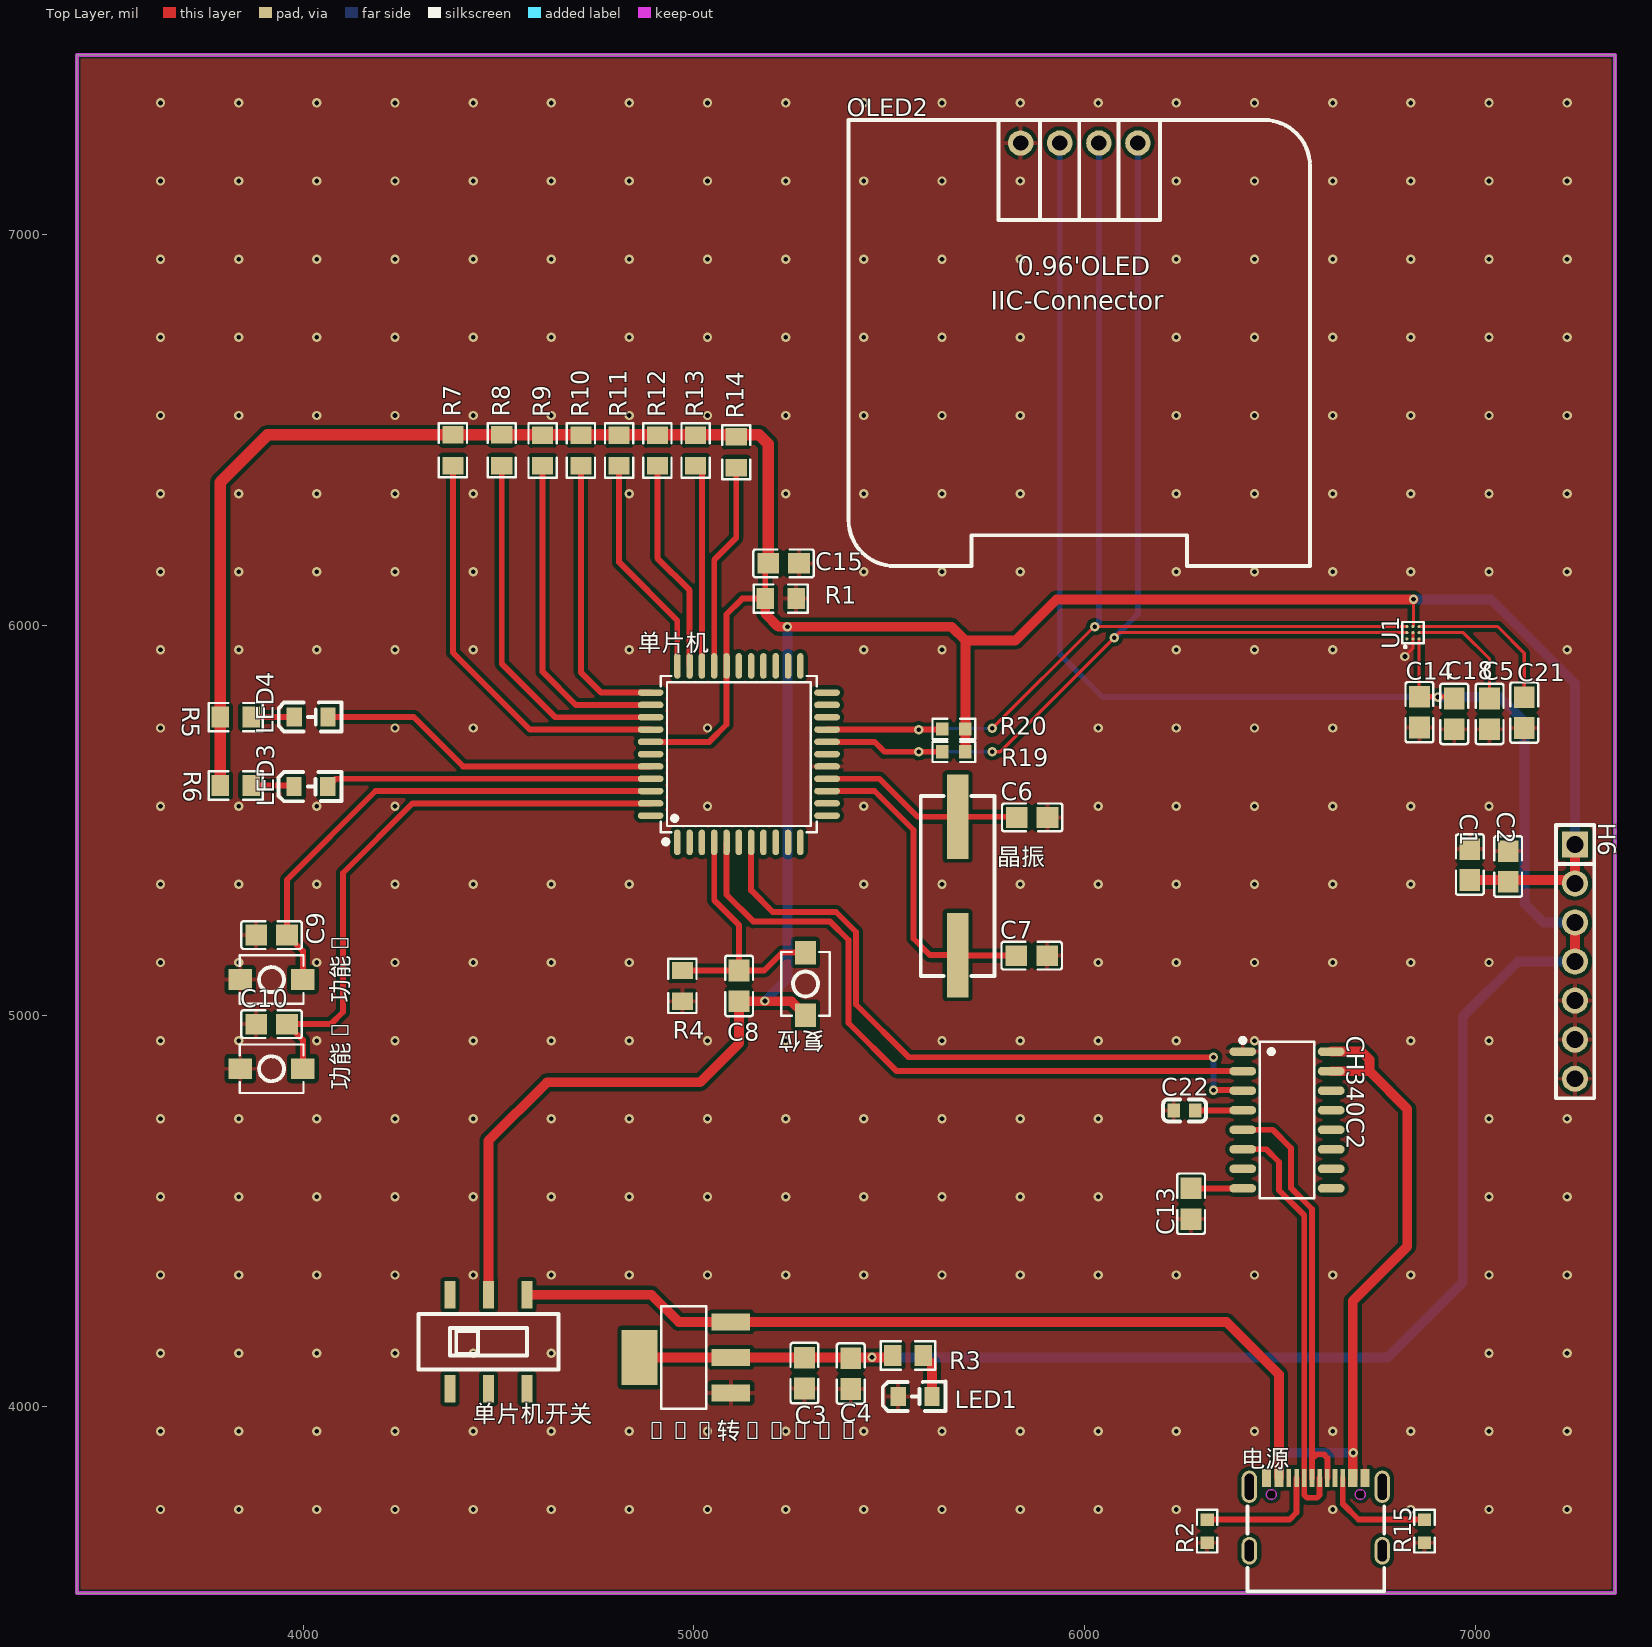
[diagram p0: Top Layer view]
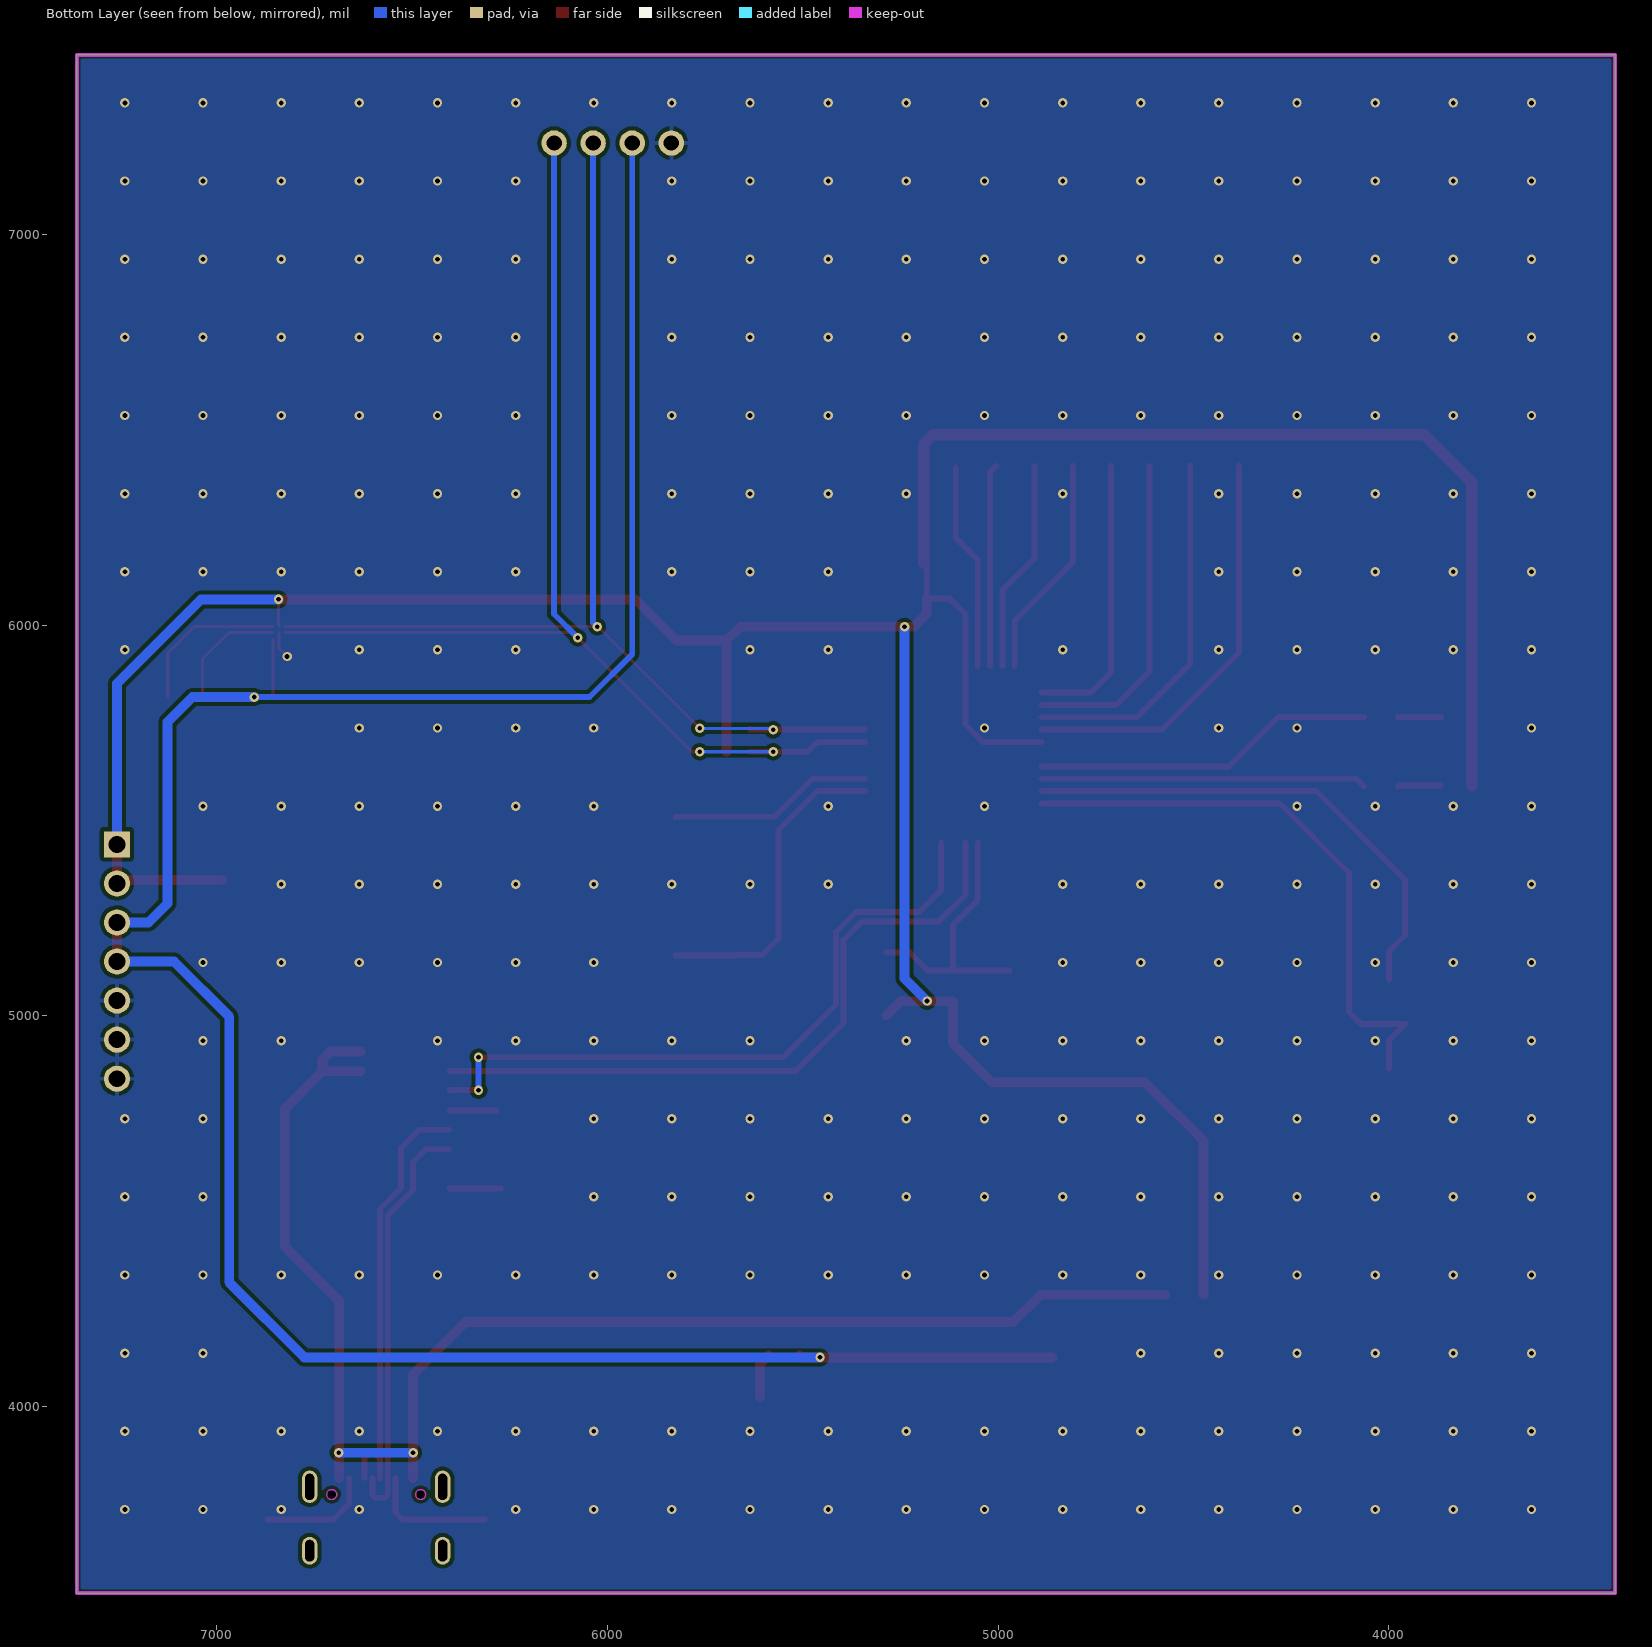
[diagram p1: Bottom Layer view, seen from below]
# Altium PCB MISC51448.pcbdoc
Units mil, origin at the board's own origin, x right, y up, seen from the top; angles counter-clockwise.
Board outline 3937.01 x 3937.01 mil, 2 copper layers (Top Layer, Bottom Layer), stack 62.206 mil thick; 48 components, 56 nets, 186 pads, 307 vias.

## Layer stack, top to bottom
Top Solder Mask Layer: solder mask 0.394, Dk 3.3
Top Layer: signal copper 1.379
Dielectric1: surface 59.449, FR4, Dk 4.5
Bottom Layer: signal copper 1.378
Bottom Solder Mask Layer: solder mask 0.394, Dk 3.3

## Board outline
3420.99,7459.65 3420.99,3522.65 7358,3522.65 7358,7459.65

## Design rules (kind name [scope] priority, off if disabled: settings)
BoardOutlineClearance copperThickness2oz_1 [All] p2 off: genericclearance=7.99 ignorepadtopadclearanceinfootprint=FALSE except(0: Arc-SplitContinuation Track-SplitContinuation SMDPad-SplitContinuation THPad-SplitContinuation Via-SplitContinuation Fill-SplitContinuation Region-SplitContinuation Poly-SplitContinuation Text-SplitContinuation Hole-SplitContinuation; 5.98: Arc-CutoutEdge SMDPad-CutoutEdge THPad-CutoutEdge Via-CutoutEdge Fill-CutoutEdge Region-CutoutEdge Text-CutoutEdge; 6.93: Hole-OutlineEdge Hole-CutoutEdge; 10: Poly-OutlineEdge Poly-CutoutEdge; 11.81: Arc-OutlineEdge Track-OutlineEdge SMDPad-OutlineEdge THPad-OutlineEdge Via-OutlineEdge Fill-OutlineEdge Region-OutlineEdge Text-OutlineEdge Track-CutoutEdge)
BoardOutlineClearance Plane_innerPlane_1 [All] p4 off: genericclearance=4.02 ignorepadtopadclearanceinfootprint=FALSE except(0: Arc-SplitContinuation Track-SplitContinuation SMDPad-SplitContinuation THPad-SplitContinuation Via-SplitContinuation Fill-SplitContinuation Region-SplitContinuation Poly-SplitContinuation Text-SplitContinuation Hole-SplitContinuation; 6: SMDPad-CutoutEdge THPad-CutoutEdge Via-CutoutEdge Fill-CutoutEdge Region-CutoutEdge Text-CutoutEdge; 6.93: Hole-OutlineEdge Hole-CutoutEdge; 10: Poly-OutlineEdge Poly-CutoutEdge; 11.8: Arc-OutlineEdge Track-OutlineEdge SMDPad-OutlineEdge THPad-OutlineEdge Via-OutlineEdge Fill-OutlineEdge Region-OutlineEdge Text-OutlineEdge; 11.81: Arc-CutoutEdge Track-CutoutEdge)
BoardOutlineClearance Copper_copperRegion_1 [All] p6 off: genericclearance=4.02 ignorepadtopadclearanceinfootprint=FALSE except(0: Arc-SplitContinuation Track-SplitContinuation SMDPad-SplitContinuation THPad-SplitContinuation Via-SplitContinuation Fill-SplitContinuation Region-SplitContinuation Poly-SplitContinuation Text-SplitContinuation Hole-SplitContinuation; 6: SMDPad-CutoutEdge THPad-CutoutEdge Via-CutoutEdge Fill-CutoutEdge Region-CutoutEdge Text-CutoutEdge; 6.93: Hole-OutlineEdge Hole-CutoutEdge; 10: Poly-OutlineEdge Poly-CutoutEdge; 11.8: Arc-OutlineEdge Track-OutlineEdge SMDPad-OutlineEdge THPad-OutlineEdge Via-OutlineEdge Fill-OutlineEdge Region-OutlineEdge Text-OutlineEdge; 11.81: Arc-CutoutEdge Track-CutoutEdge)
BoardOutlineClearance copperThickness1oz_1 [All] p8: genericclearance=4.02 ignorepadtopadclearanceinfootprint=FALSE except(0: Arc-SplitContinuation Track-SplitContinuation SMDPad-SplitContinuation THPad-SplitContinuation Via-SplitContinuation Fill-SplitContinuation Region-SplitContinuation Poly-SplitContinuation Text-SplitContinuation Hole-SplitContinuation; 6: SMDPad-CutoutEdge THPad-CutoutEdge Via-CutoutEdge Fill-CutoutEdge Region-CutoutEdge Text-CutoutEdge; 6.93: Hole-OutlineEdge Hole-CutoutEdge; 10: Poly-OutlineEdge Poly-CutoutEdge; 11.8: Arc-OutlineEdge Track-OutlineEdge SMDPad-OutlineEdge THPad-OutlineEdge Via-OutlineEdge Fill-OutlineEdge Region-OutlineEdge Text-OutlineEdge; 11.81: Arc-CutoutEdge Track-CutoutEdge)
Clearance copperThickness2oz [All] p1 off: gap=7.99 ignorepadtopadclearanceinfootprint=FALSE except(5.98: SMDPad-Track SMDPad-SMDPad THPad-Track SMDPad-THPad THPad-THPad Track-Via SMDPad-Via THPad-Via Via-Via Fill-Track Region-Track Fill-SMDPad Region-SMDPad Fill-THPad Region-THPad Fill-Via Region-Via Fill-Fill Fill-Region Region-Region Arc-Track Arc-SMDPad Arc-THPad Arc-Via Fill-Arc Region-Arc Arc-Arc Text-Track SMDPad-Text Text-THPad Text-Via Fill-Text Region-Text Arc-Text Text-Text; 6.93: Hole-Track Hole-SMDPad Hole-THPad Hole-Via Fill-Hole Region-Hole Hole-Arc Hole-Text; 10: Poly-Track Poly-SMDPad Poly-THPad Poly-Via Poly-Fill Poly-Region Poly-Poly Poly-Arc Poly-Text Poly-Hole)
Clearance Plane_innerPlane [All] p3 off: gap=4.02 ignorepadtopadclearanceinfootprint=FALSE except(4.33: SMDPad-Track SMDPad-SMDPad SMDPad-THPad; 5.98: THPad-Track THPad-THPad Track-Via SMDPad-Via THPad-Via Via-Via Fill-Track Region-Track Fill-SMDPad Region-SMDPad Fill-THPad Region-THPad Fill-Via Region-Via Fill-Fill Fill-Region Region-Region; 6: Arc-Track Arc-SMDPad Arc-THPad Arc-Via Fill-Arc Region-Arc Arc-Arc Text-Track SMDPad-Text Text-THPad Text-Via Fill-Text Region-Text Arc-Text Text-Text; 6.93: Hole-Track Hole-SMDPad Hole-THPad Hole-Via Fill-Hole Region-Hole Hole-Arc Hole-Text; 10: Poly-Track Poly-SMDPad Poly-THPad Poly-Via Poly-Fill Poly-Region Poly-Poly Poly-Arc Poly-Text Poly-Hole)
Clearance Copper_copperRegion [All] p5 off: gap=4.02 ignorepadtopadclearanceinfootprint=FALSE except(4.33: SMDPad-Track SMDPad-SMDPad SMDPad-THPad; 5.98: THPad-Track THPad-THPad Track-Via SMDPad-Via THPad-Via Via-Via Fill-Track Region-Track Fill-SMDPad Region-SMDPad Fill-THPad Region-THPad Fill-Via Region-Via Fill-Fill Fill-Region Region-Region; 6: Arc-Track Arc-SMDPad Arc-THPad Arc-Via Fill-Arc Region-Arc Arc-Arc Text-Track SMDPad-Text Text-THPad Text-Via Fill-Text Region-Text Arc-Text Text-Text; 6.93: Hole-Track Hole-SMDPad Hole-THPad Hole-Via Fill-Hole Region-Hole Hole-Arc Hole-Text; 10: Poly-Track Poly-SMDPad Poly-THPad Poly-Via Poly-Fill Poly-Region Poly-Poly Poly-Arc Poly-Text Poly-Hole)
Clearance copperThickness1oz [All] p7: gap=4.02 ignorepadtopadclearanceinfootprint=FALSE except(4.33: SMDPad-Track SMDPad-SMDPad SMDPad-THPad; 5.98: THPad-Track THPad-THPad Track-Via SMDPad-Via THPad-Via Via-Via Fill-Track Region-Track Fill-SMDPad Region-SMDPad Fill-THPad Region-THPad Fill-Via Region-Via Fill-Fill Fill-Region Region-Region; 6: Arc-Track Arc-SMDPad Arc-THPad Arc-Via Fill-Arc Region-Arc Arc-Arc Text-Track SMDPad-Text Text-THPad Text-Via Fill-Text Region-Text Arc-Text Text-Text; 6.93: Hole-Track Hole-SMDPad Hole-THPad Hole-Via Fill-Hole Region-Hole Hole-Arc Hole-Text; 10: Poly-Track Poly-SMDPad Poly-THPad Poly-Via Poly-Fill Poly-Region Poly-Poly Poly-Arc Poly-Text Poly-Hole)
DiffPairsRouting differentialPair [All] p1: maxlimit=6 minlimit=6 mostfreqgap=6 toplayer_minwidth=5 toplayer_prefwidth=10 toplayer_maxwidth=100 toplayer_mingap=6 toplayer_prefgap=6 toplayer_maxgap=6 bottomlayer_minwidth=5 bottomlayer_prefwidth=10 bottomlayer_maxwidth=100 bottomlayer_mingap=6 bottomlayer_prefgap=6 bottomlayer_maxgap=6 maxuncoupledlength=10
HoleToHoleClearance otherClearance [All] p1: gap=11.81 allowstackedmicrovias=TRUE
Length netLength [All] p1: minlimit=0 maxlimit=0
PasteMaskExpansion pasteMaskExpansion [All] p1: expansion=0
PlaneConnect innerPlane [All] p1: planeconnectstyle=Relief reliefexpansion=20 reliefentries=4 reliefconductorwidth=10 reliefairgap=10
PolygonConnect copperRegion [(InNet('GND'))] p1: connectstyle=Relief reliefconductorwidth=10 reliefentries=4 polygonreliefangle="90 Angle" airgapwidth=10 via.connectstyle=Relief via.reliefconductorwidth=10 via.reliefentries=4 via.polygonreliefangle="90 Angle" via.airgapwidth=10
RoutingVias viaSize [All] p1: holewidth=12.01 width=24.02 viastyle="Through Hole" minholewidth=11.81 minwidth=19.68 maxholewidth=248.03 maxwidth=393.7
SolderMaskExpansion solderMaskExpansion [IsVia] p1: expansion=-1000 istentingtop=TRUE
SolderMaskExpansion solderMaskExpansion [All] p2: expansion=2 istentingtop=FALSE
Width copperThickness2oz_2 [All] p1 off: maxlimit=100 minlimit=8 preferedwidth=10
Width copperThickness1oz_2 [All] p2: maxlimit=100 minlimit=5 preferedwidth=10

## Components (designator, comment, footprint, x,y, rotation, side; value= is the part's Value field where it differs from the comment)
+5v转+3.3v "AMS1117-3.3" SOT-223-3_L6.5-W3.4-P2.30-LS7.0-BR 4978.16,4125.83 r0 top (schematic designator +5vת+3.3v)
C1 "10UF" C0805 6986.23,5387.32 r270 top
C2 "100nF" C0805 7084.29,5382.37 r270 top
C3 "100nF" C0805 5283.16,4085.83 r90 top
C4 "10UF" C0805 5401.65,4084.52 r90 top
C5 "2.2uF" C0805 7036.7,5772.95 r270 top
C6 "22PF" C0805 5866,5508 r0 top
C7 "22PF" C0805 5864.87,5154.16 r0 top
C8 "10UF" C0805 5115.91,5076.74 r90 top
C9 "0.1uf" C0805 3919.2,5206.85 r0 top
C10 "0.1uf" C0805 3919.2,4978.82 r0 top
C13 "0.1UF" C0805 6272.61,4519.17 r90 top
C14 "10UF" C0805 6857.12,5777.32 r270 top
C15 "0.1uF" C0805 5229.65,6158.23 r180 top
C18 "0.1UF" C0805 6946.34,5772.95 r90 top
C21 "0.1UF" C0805 7125.53,5776.17 r90 top
C22 "100nF" C0603 6256,4758 r0 top
CH340C2 "CH340C" SOP-16_L10.0-W3.9-P1.27-LS6.0-BL 6518.14,4733.56 r270 top
H6 "" HDR-TH_7P-P2.54-V-M 7255.44,5139.1 r270 top
LED1 "" LED_0805 5568.16,4025.83 r0 top
LED3 "" LED_0805 4021.97,5586.62 r0 top
LED4 "" LED_0805 4022.41,5764.73 r0 top
OLED2 "0.96OLED_4P_MODULE_JX" 0.96OLED_4P 5986.62,7234.06 r0 top
R1 "1K" R0805 5222.29,6068.02 r180 top
R2 "5.1K" R0603 6313.91,3681.25 r90 top
R3 "1K" R0805 5548.16,4130.83 r0 top
R4 "10K" R0805 4970.91,5076.74 r90 top
R5 "1K" R0805 3827.41,5764.73 r180 top
R6 "1K" R0805 3827.41,5589.73 r180 top
R7 "10K" R0805 4383.51,6447.72 r90 top
R8 "10K" R0805 4508.51,6447.72 r90 top
R9 "10K" R0805 4613.01,6447.1 r90 top
R10 "10K" R0805 4710.91,6447.1 r90 top
R11 "10K" R0805 4808.81,6447.1 r90 top
R12 "10K" R0805 4906.7,6447.1 r90 top
R13 "10K" R0805 5004.6,6447.1 r90 top
R14 "10K" R0805 5108.51,6442.72 r90 top
R15 "5.1K" R0603 6870.09,3681.25 r90 top
R19 "4.7K" R0603 5665.36,5675.95 r180 top
R20 "4.7K" R0603 5665.36,5734.18 r180 top
U1 "BMM350" WLCSP-9_L1.3-W1.3-R3-C3-P0.40-TL 6840.74,5980.81 r90 top
功能1 "轻触按键3*4*H" SW-SMD_L4.0-W2.9-LS5.0 3919.2,5092.84 r180 top
功能2 "轻触按键3*4*H" SW-SMD_L4.0-W2.9-LS5.0 3919.2,4864.81 r180 top
单片机 "STC89C52RC-40I-LQFP44" LQFP-44_L10.0-W10.0-P0.80-LS12.0-BL 5115.2,5669.93 r0 top
单片机开关 "SS-3235S-L1" SW-SMD_SS-3235S-LX 4474.69,4166.03 r180 top
复位 "轻触按键3*4*H" SW-SMD_L4.0-W2.9-LS5.0 5285.91,5081.74 r270 top
晶振 "12MHz" CRYSTAL-SMD_L11.4-W4.7-LS12.7 5675.2,5332.57 r270 top
电源 "Type-C" USB-C-SMD_TYPE-C16PIN 6592,3724.3 r0 top

## Footprints (in the part's own frame and the unit in brackets; to place one, negate y for a bottom-side part, rotate by r counter-clockwise, add the part's x,y. Pads: shape width x height; smd on the part's side, far side on the other; paste and mask are expansions set on the pad)
0.96OLED_4P [mm]
  round 1.65 hole 1 copper offset 0,0: 1(-3.81,-0.001) 2(-1.27,0.002) 3(1.27,0.002) 4(3.81,0.002)
  silkscreen extent -15,-27.5 15,1.5
C0603 [mm]
  rect 0.8x0.9 smd: 1(-0.7,0) 2(0.7,0)
  silkscreen extent -1.39,-0.71 1.39,0.71
C0805 [mm]
  rect 1.41x1.35 smd paste-100 mask+0.051: 1(-1,0) 2(1,0)
  silkscreen extent -1.96,-0.9 1.96,0.9
CRYSTAL-SMD_L11.4-W4.7-LS12.7 [mm]
  rect 5.5x1.4 smd: 1(-4.5,0) 2(4.5,0)
  silkscreen extent -5.85,-2.4 5.85,2.4
HDR-TH_7P-P2.54-V-M [mm]
  rect 1.7x1.7 hole 1.1: 1(-7.62,0)
  round 1.7 hole 1.1: 2(-5.08,0) 3(-2.54,0) 4(0,0) 5(2.54,0) 6(5.08,0) 7(7.62,0)
  silkscreen extent -8.89,-1.25 8.89,1.25
LED_0805 [mm]
  rect 1x1.25 smd paste+0 mask+0.051: 1(-1.15,0.005) 2(1.05,0.005)
  silkscreen extent -2.15,-0.94 1.93,0.97
LQFP-44_L10.0-W10.0-P0.80-LS12.0-BL [mm]
  oval 0.42x1.67 smd: 1(-4,-5.735) 2(-3.2,-5.735) 3(-2.4,-5.735) 4(-1.6,-5.735) 5(-0.8,-5.735) 6(0,-5.735) 7(0.8,-5.735) 8(1.6,-5.735) 9(2.4,-5.735) 10(3.2,-5.735) 11(4,-5.735) 23(4,5.735) 24(3.2,5.735) 25(2.4,5.735) 26(1.6,5.735) 27(0.8,5.735) 28(0,5.735) 29(-0.8,5.735) 30(-1.6,5.735) 31(-2.4,5.735) 32(-3.2,5.735) 33(-4,5.735)
  oval 1.67x0.42 smd: 12(5.735,-4) 13(5.735,-3.2) 14(5.735,-2.4) 15(5.735,-1.6) 16(5.735,-0.8) 17(5.735,0) 18(5.735,0.8) 19(5.735,1.6) 20(5.735,2.4) 21(5.735,3.2) 22(5.735,4) 34(-5.735,4) 35(-5.735,3.2) 36(-5.735,2.4) 37(-5.735,1.6) 38(-5.735,0.8) 39(-5.735,0) 40(-5.735,-0.8) 41(-5.735,-1.6) 42(-5.735,-2.4) 43(-5.735,-3.2) 44(-5.735,-4)
  silkscreen extent -5.08,-5.85 5.08,5.08
R0603 [mil]
  rect 31.75x34.02 smd paste-3937.01 mask+2: 1(-29.66,0) 2(29.66,0)
  silkscreen extent -55,-26 55,26
R0805 [mm]
  rect 1.133x1.377 smd paste-100 mask+0.051: 1(-1,0) 2(1,0)
  silkscreen extent -1.76,-0.92 1.76,0.92
SOP-16_L10.0-W3.9-P1.27-LS6.0-BL [mm]
  oval 0.56x1.745 smd: 1(-4.445,-2.872) 2(-3.175,-2.872) 3(-1.905,-2.872) 4(-0.635,-2.872) 5(0.635,-2.872) 6(1.905,-2.872) 7(3.175,-2.872) 8(4.445,-2.872) 9(4.445,2.872) 10(3.175,2.872) 11(1.905,2.872) 12(0.635,2.872) 13(-0.635,2.872) 14(-1.905,2.872) 15(-3.175,2.872) 16(-4.445,2.872)
  silkscreen extent -5.33,-3.02 5.08,1.77
SOT-223-3_L6.5-W3.4-P2.30-LS7.0-BR [mm]
  rect 2.5x1.1 smd: 1(2.97,-2.3) 2(2.97,0) 3(2.97,2.3)
  rect 2.34x3.6 smd: 4(-2.97,0)
  silkscreen extent -1.57,-3.33 1.37,3.33
SW-SMD_L4.0-W2.9-LS5.0 [mm]
  rect 1.53x1.36 smd: 1(-2.035,0) 2(2.035,0)
  silkscreen extent -2.08,-1.58 2.08,1.58
SW-SMD_SS-3235S-LX [mm]
  rect 0.7x1.8 smd: 1(-2.5,3.05) 2(0,3.05) 3(2.5,3.05) 4(-2.5,-3.05) 5(0,-3.05) 6(2.5,-3.05)
  silkscreen extent -4.55,-1.8 4.55,1.8
USB-C-SMD_TYPE-C16PIN [mm]
  oval 1x2.1 hole 0.6 slot 1.7 at 90 deg: 1(-4.32,1.787) 2(4.32,1.787)
  oval 1x1.8 hole 0.6 slot 1.4 at 90 deg: 3(-4.32,-2.362) 4(4.32,-2.362)
  rect 0.6x1.15 smd paste-100 mask+0.051: A1B12(-3.2,2.362) A4B9(-2.4,2.362) B1A12(3.2,2.362) B4A9(2.4,2.362)
  rect 0.3x1.15 smd paste-100 mask+0.051: A5(-1.25,2.362) A6(-0.25,2.362) A7(0.25,2.362) A8(1.25,2.362) B5(1.75,2.362) B6(0.75,2.362) B7(-0.75,2.362) B8(-1.75,2.362)
  Board Outline Layer circle w0.003: c2.89,1.288 r0.325
  Board Outline Layer circle w0.003: c-2.89,1.288 r0.325
  Board Outline Layer region: 3.215,1.288 3.183,1.147 3.093,1.034 2.962,0.971 2.818,0.971 2.687,1.034 2.597,1.147 2.565,1.288 2.565,1.288 2.597,1.429 2.687,1.542 2.818,1.605 2.962,1.605 3.093,1.542 3.183,1.429 3.215,1.288
  Board Outline Layer region: 3.215,1.288 3.206,1.21 3.178,1.137 3.133,1.073 3.075,1.021 3.005,0.984 2.929,0.965 2.851,0.965 2.775,0.984 2.705,1.021 2.647,1.073 2.602,1.137 2.574,1.21 2.565,1.288 2.574,1.366 2.602,1.439 2.647,1.504 2.705,1.555 2.775,1.592 2.851,1.611 2.929,1.611 3.005,1.592 3.075,1.555 3.133,1.504 3.178,1.439 3.206,1.366
  Board Outline Layer region: -2.565,1.288 -2.597,1.147 -2.687,1.034 -2.818,0.971 -2.962,0.971 -3.093,1.034 -3.183,1.147 -3.215,1.288 -3.215,1.288 -3.183,1.429 -3.093,1.542 -2.962,1.605 -2.818,1.605 -2.687,1.542 -2.597,1.429 -2.565,1.288
  Board Outline Layer region: -2.565,1.288 -2.574,1.21 -2.602,1.137 -2.647,1.073 -2.705,1.021 -2.775,0.984 -2.851,0.965 -2.929,0.965 -3.005,0.984 -3.075,1.021 -3.133,1.073 -3.178,1.137 -3.206,1.21 -3.215,1.288 -3.206,1.366 -3.178,1.439 -3.133,1.504 -3.075,1.555 -3.005,1.592 -2.929,1.611 -2.851,1.611 -2.775,1.592 -2.705,1.555 -2.647,1.504 -2.602,1.439 -2.574,1.366
  Multi-Layer board cut-out: 3.215,1.288 3.183,1.147 3.093,1.034 2.962,0.971 2.818,0.971 2.687,1.034 2.597,1.147 2.565,1.288 2.565,1.288 2.597,1.429 2.687,1.542 2.818,1.605 2.962,1.605 3.093,1.542 3.183,1.429 3.215,1.288
  Multi-Layer board cut-out: -2.565,1.288 -2.597,1.147 -2.687,1.034 -2.818,0.971 -2.962,0.971 -3.093,1.034 -3.183,1.147 -3.215,1.288 -3.215,1.288 -3.183,1.429 -3.093,1.542 -2.962,1.605 -2.818,1.605 -2.687,1.542 -2.597,1.429 -2.565,1.288
  silkscreen extent -4.45,-5 4.45,0.52
WLCSP-9_L1.3-W1.3-R3-C3-P0.40-TL [mm]
  round 0.2 smd paste-100 mask+0.051: A1(-0.4,0.4) A2(0,0.4) A3(0.4,0.4) B1(-0.4,0) B2(0,0) B3(0.4,0) C1(-0.4,-0.4) C2(0,-0.4) C3(0.4,-0.4)
  silkscreen extent -1,-0.7 0.7,0.7

## Via types
v1: diameter 24.02, hole 12, Top Layer to Bottom Layer, 307 vias

## Nets (pads, with @x,y where several pads share a name; then routed paths per layer and width w, separated by ;. In a path a pad name is that pad's centre, name@x,y a point inside that pad or via, vN(x,y) a via of type N, cw(c..) or ccw(c..) an arc to the next point about the centre after c; other vN are vias at no path point)
3.3V: +5v转+3.3v.2 +5v转+3.3v.4 C3.2 C4.2 C14.1 C18.2 H6.3 H6.4 OLED2.2 R3.1 U1.C1 | length 6790.3
  Top Layer w8: U1.C1 6856.49,5817.32 C14.1
  Top Layer w15: C14.1 6941.97,5816.69 C18.2
  Top Layer w25: +5v转+3.3v.4 +5v转+3.3v.2 5503.79,4125.83 R3.1 ; H6.4 H6.3
  Bottom Layer w15: OLED2.2 5936.62,5925.38 6046,5816 v1(6904,5816)
  Bottom Layer w25: v1(5456,4126) 6776,4126 6968,4318 6968,4998 7109.1,5139.1 H6.4 ; v1(6904,5816) 7062,5816 7126,5752 7126,5288 7174.9,5239.1 H6.3
$1N1944: LED4.1 R5.1 | length 110.4
  Top Layer w15: R5.1 3976.93,5764.73 LED4.1
$1N1945: LED3.1 R6.1 | length 111.1
  Top Layer w15: R6.1 3973.79,5589.73 LED3.1
$1N2954: LED1.2 R3.2 | length 113.9
  Top Layer w25: R3.2 5609.5,4108.87 LED1.2
$1N3992: C22.2 CH340C2.4 | length 121.7
  Top Layer w15: C22.2 6404.49,4758 CH340C2.4
$1N3994: R15.2 电源.B5 | length 292
  Top Layer w15: 电源.B5 6660.9,3751.1 6701.09,3710.91 R15.2
$1N3995: R2.2 电源.A5 | length 324.8
  Top Layer w15: R2.2 6524.91,3710.91 6542.79,3728.79 电源.A5
$1N3998: C21.2 U1.C3 | length 410.2
  Top Layer w8: U1.C3 7057.44,5996.56 7125.53,5928.47 C21.2
$1N3999: C5.1 U1.C2 | length 309.2
  Top Layer w8: U1.C2 6969.19,5980.81 7036.7,5913.3 C5.1
$1N4005: CH340C2.6 电源.A7 电源.B7 | length 1074.2
  Top Layer w15: CH340C2.6 6465.44,4658.56 6498,4626 6498,4554 6562.47,4489.53 电源.B7 6562.47,3773.53 6569.16,3766.84 6595,3766.84 6601.84,3773.67 电源.A7
$1N4006: CH340C2.5 电源.A6 电源.B6 | length 1108.7
  Top Layer w15: CH340C2.5 6481.44,4708.56 6528,4662 6528,4560 6582.16,4505.84 6582.16,3866.16 ; 电源.A6 6582.16,3866.16 ; 电源.B6 6621.53,3868.47 6612,3878 6594,3878 6582.16,3866.16
$1N4007: C13.2 CH340C2.8 | length 132.4
  Top Layer w15: C13.2@6272.63,4558.56 CH340C2.8
"+ 5V_S": +5v转+3.3v.3 CH340C2.15 CH340C2.16 单片机开关.4 电源.A4B9 电源.B4A9 | length 3838.1
  Top Layer w25: 单片机开关.4 4891.89,4286.11 4961.62,4216.38 +5v转+3.3v.3 6363.62,4216.38 6497.51,4082.49 v1(6497.51,3882) 电源.A4B9 ; CH340C2.15 6729.44,4858.56 ; CH340C2.16 6709.44,4908.56 6729.44,4888.56 6729.44,4858.56 ; 电源.B4A9 6686.49,4270.49 6826,4410 6826,4762 6729.44,4858.56
  Bottom Layer w25: v1(6497.51,3882) v1(6688,3882)
"+ 5V_SW": C1.2 C2.2 C8.1 C15.2 H6.1 H6.2 R1.2 R5.2 R6.2 R7.2 R8.2 R9.2 R10.2 R11.2 R12.2 R13.2 R14.2 R19.1 R20.1 U1.B3 单片机.29 单片机.38 单片机开关.5 复位.2 | length 9072.7
  Top Layer w8: U1.B3 6842,5997.82 v1(6842,6066)
  Top Layer w15: 单片机.38 5039.43,5701.43 5083.7,5745.7 单片机.29 5083.7,6027.96 5123.77,6068.02 R1.2 5182.92,6150.86 C15.2
  Top Layer w25: 单片机开关.5 4474.69,4680.69 4624,4830 5016,4830 5115.91,4929.91 C8.1 5250.16,5037.37 复位.2 ; R1.2 5182.92,6029.08 5216,5996 v1(5239.56,5996) 5660,5996 5695.02,5960.98 ; R19.1 R20.1 5695.02,5960.98 ; v1(6842,6066) 5928,6066 5822.98,5960.98 5695.02,5960.98 ; C1.2 7246.6,5347.95 H6.2 H6.1
  Top Layer w30: R6.2 R5.2 3788.04,6366.04 3909.09,6487.09 R7.2 R8.2 5166.91,6487.09 5190.28,6463.72 C15.2
  Bottom Layer w25: v1(5182,5038) 5239.56,5095.56 v1(5239.56,5996) ; v1(6842,6066) 7040,6066 7255.44,5850.56 H6.1
GND: +5v转+3.3v.1 C1.1 C2.1 C3.1 C4.1 C5.2 C6.2 C7.2 C9.1 C10.1 C13.1 C14.2 C15.1 C18.1 C21.1 C22.1 CH340C2.1 H6.5 H6.6 H6.7 LED1.1 OLED2.1 R1.1 R2.1 R4.1 R15.1 U1.B1 U1.B2 功能1.2 功能2.2 单片机.16 电源.B1A12 | length 69.4
  Top Layer w8: v1(6820,5920) 6840.74,5940.74 U1.B1 U1.B2
  other v1: 3635.09,3736.75 3835.09,3736.75 4035.09,3736.75 4235.09,3736.75 4435.09,3736.75 4635.09,3736.75 4835.09,3736.75 5035.09,3736.75 5235.09,3736.75 5435.09,3736.75 5635.09,3736.75 5835.09,3736.75 6035.09,3736.75 6235.09,3736.75 6635.09,3736.75 6835.09,3736.75 7035.09,3736.75 7235.09,3736.75 3635.09,3936.75 3835.09,3936.75 4035.09,3936.75 4235.09,3936.75 4435.09,3936.75 4635.09,3936.75 4835.09,3936.75 5035.09,3936.75 5235.09,3936.75 5435.09,3936.75 5635.09,3936.75 5835.09,3936.75 6035.09,3936.75 6235.09,3936.75 6435.09,3936.75 6635.09,3936.75 6835.09,3936.75 7035.09,3936.75 7235.09,3936.75 3635.09,4136.75 3835.09,4136.75 4035.09,4136.75 4235.09,4136.75 4435.09,4136.75 4635.09,4136.75 7035.09,4136.75 7235.09,4136.75 3635.09,4336.75 3835.09,4336.75 4035.09,4336.75 4235.09,4336.75 4435.09,4336.75 4635.09,4336.75 4835.09,4336.75 5035.09,4336.75 5235.09,4336.75 5435.09,4336.75 5635.09,4336.75 5835.09,4336.75 6035.09,4336.75 6235.09,4336.75 6435.09,4336.75 6635.09,4336.75 6835.09,4336.75 7035.09,4336.75 7235.09,4336.75 3635.09,4536.75 3835.09,4536.75 4035.09,4536.75 4235.09,4536.75 4435.09,4536.75 4635.09,4536.75 4835.09,4536.75 5035.09,4536.75 5235.09,4536.75 5435.09,4536.75 5635.09,4536.75 5835.09,4536.75 6035.09,4536.75 7035.09,4536.75 7235.09,4536.75 3635.09,4736.75 3835.09,4736.75 4035.09,4736.75 4235.09,4736.75 4435.09,4736.75 4635.09,4736.75 4835.09,4736.75 5035.09,4736.75 5235.09,4736.75 5435.09,4736.75 5635.09,4736.75 5835.09,4736.75 6035.09,4736.75 7035.09,4736.75 7235.09,4736.75 3635.09,4936.75 3835.09,4936.75 4035.09,4936.75 4235.09,4936.75 4435.09,4936.75 4635.09,4936.75 4835.09,4936.75 5035.09,4936.75 5235.09,4936.75 5635.09,4936.75 5835.09,4936.75 6035.09,4936.75 6235.09,4936.75 6435.09,4936.75 6835.09,4936.75 7035.09,4936.75 3635.09,5136.75 3835.09,5136.75 4035.09,5136.75 4235.09,5136.75 4435.09,5136.75 4635.09,5136.75 4835.09,5136.75 6035.09,5136.75 6235.09,5136.75 6435.09,5136.75 6635.09,5136.75 6835.09,5136.75 7035.09,5136.75 3635.09,5336.75 3835.09,5336.75 4035.09,5336.75 4235.09,5336.75 4435.09,5336.75 4635.09,5336.75 4835.09,5336.75 5435.09,5336.75 5635.09,5336.75 5835.09,5336.75 6035.09,5336.75 6235.09,5336.75 6435.09,5336.75 6635.09,5336.75 6835.09,5336.75 3635.09,5536.75 3835.09,5536.75 4035.09,5536.75 4235.09,5536.75 5035.09,5536.75 5435.09,5536.75 6035.09,5536.75 6235.09,5536.75 6435.09,5536.75 6635.09,5536.75 6835.09,5536.75 7035.09,5536.75 3635.09,5736.75 4235.09,5736.75 4435.09,5736.75 5035.09,5736.75 6035.09,5736.75 6235.09,5736.75 6435.09,5736.75 6635.09,5736.75 3635.09,5936.75 3835.09,5936.75 4035.09,5936.75 4235.09,5936.75 4435.09,5936.75 4835.09,5936.75 5435.09,5936.75 5635.09,5936.75 6235.09,5936.75 6435.09,5936.75 6635.09,5936.75 7235.09,5936.75 3635.09,6136.75 3835.09,6136.75 4035.09,6136.75 4235.09,6136.75 4435.09,6136.75 5435.09,6136.75 5635.09,6136.75 5835.09,6136.75 6235.09,6136.75 6435.09,6136.75 6635.09,6136.75 6835.09,6136.75 7035.09,6136.75 7235.09,6136.75 3635.09,6336.75 3835.09,6336.75 4035.09,6336.75 4235.09,6336.75 4435.09,6336.75 4835.09,6336.75 5235.09,6336.75 5435.09,6336.75 5635.09,6336.75 5835.09,6336.75 6235.09,6336.75 6435.09,6336.75 6635.09,6336.75 6835.09,6336.75 7035.09,6336.75 7235.09,6336.75 3635.09,6536.75 3835.09,6536.75 4035.09,6536.75 4235.09,6536.75 4435.09,6536.75 4635.09,6536.75 4835.09,6536.75 5035.09,6536.75 5235.09,6536.75 5435.09,6536.75 5635.09,6536.75 5835.09,6536.75 6235.09,6536.75 6435.09,6536.75 6635.09,6536.75 6835.09,6536.75 7035.09,6536.75 7235.09,6536.75 3635.09,6736.75 3835.09,6736.75 4035.09,6736.75 4235.09,6736.75 4435.09,6736.75 4635.09,6736.75 4835.09,6736.75 5035.09,6736.75 5235.09,6736.75 5435.09,6736.75 5635.09,6736.75 5835.09,6736.75 6235.09,6736.75 6435.09,6736.75 6635.09,6736.75 6835.09,6736.75 7035.09,6736.75 7235.09,6736.75 3635.09,6936.75 3835.09,6936.75 4035.09,6936.75 4235.09,6936.75 4435.09,6936.75 4635.09,6936.75 4835.09,6936.75 5035.09,6936.75 5235.09,6936.75 5435.09,6936.75 5635.09,6936.75 5835.09,6936.75 6235.09,6936.75 6435.09,6936.75 6635.09,6936.75 6835.09,6936.75 7035.09,6936.75 7235.09,6936.75 3635.09,7136.75 3835.09,7136.75 4035.09,7136.75 4235.09,7136.75 4435.09,7136.75 4635.09,7136.75 4835.09,7136.75 5035.09,7136.75 5235.09,7136.75 5435.09,7136.75 5635.09,7136.75 5835.09,7136.75 6235.09,7136.75 6435.09,7136.75 6635.09,7136.75 6835.09,7136.75 7035.09,7136.75 7235.09,7136.75 3635.09,7336.75 3835.09,7336.75 4035.09,7336.75 4235.09,7336.75 4435.09,7336.75 4635.09,7336.75 4835.09,7336.75 5035.09,7336.75 5235.09,7336.75 5435.09,7336.75 5635.09,7336.75 5835.09,7336.75 6035.09,7336.75 6235.09,7336.75 6435.09,7336.75 6635.09,7336.75 6835.09,7336.75 7035.09,7336.75 7235.09,7336.75
P0.0: R7.1 单片机.37 | length 1066
  Top Layer w15: R7.1 4383.51,5929.77 4580.36,5732.92 单片机.37
P0.1: R8.1 单片机.36 | length 944.7
  Top Layer w15: R8.1 4508.51,5901.15 4645.24,5764.42 单片机.36
P0.2: R9.1 单片机.35 | length 838.4
  Top Layer w15: R9.1 4613.01,5880.98 4698.08,5795.91 单片机.35
P0.3: R10.1 单片机.34 | length 728.3
  Top Layer w15: R10.1 4710.91,5879.46 4762.96,5827.41 单片机.34
P0.4: R11.1 单片机.33 | length 573.7
  Top Layer w15: R11.1 4808.81,6161.05 4957.72,6012.13 单片机.33
P0.5: R12.1 单片机.32 | length 546.2
  Top Layer w15: R12.1 4906.7,6171.58 4989.22,6089.06 单片机.32
P0.6: R13.1 单片机.31 | length 518.7
  Top Layer w15: R13.1 5020.71,6391.62 单片机.31
P0.7: R14.1 单片机.30 | length 531
  Top Layer w15: 单片机.30 5052.21,6167.14 5108.51,6223.43 R14.1
P1.0: LED4.2 单片机.40 | length 878.1
  Top Layer w15: LED4.2 4283.07,5764.93 4409.57,5638.43 单片机.40
P1.1: LED3.2 单片机.41 | length 834.4
  Top Layer w15: LED3.2 4083.43,5606.94 单片机.41
P1.2: C9.2 功能1.1 单片机.42 | length 1297.4
  Top Layer w15: 功能1.1 3999.32,5166.1 C9.2 3958.57,5348.57 4185.44,5575.44 单片机.42
P1.3: C10.2 功能2.1 单片机.43 | length 1504.4
  Top Layer w15: 功能2.1 3999.32,4938.07 C10.2 4070.82,4978.82 4102,5010 4102,5366 4279.95,5543.95 单片机.43
P1.4: 单片机.44
P1.5: 单片机.1
P1.6: 单片机.2
P1.7: 单片机.3
P2.0: OLED2.4 R19.2 U1.A2 单片机.18 | length 2971.7
  Top Layer w8: v1(5764,5676) 5784,5676 v1(6075.94,5967.94) 6088.81,5980.81 U1.A2
  Top Layer w15: 单片机.18 5462.57,5701.43 5488.05,5675.95 v1(5576,5676) R19.2
  Bottom Layer w8: v1(5576,5676) v1(5764,5676)
  Bottom Layer w15: v1@6076,5968 6136.62,6028.62 OLED2.4
P2.1: OLED2.3 R20.2 U1.A3 单片机.19 | length 2896.3
  Top Layer w8: v1(5764,5736) 6024.56,5996.56 U1.A3
  Top Layer w15: 单片机.19 5634.44,5732.92 R20.2
  Bottom Layer w8: v1(5576,5732) 5580,5736 v1(5764,5736)
  Bottom Layer w15: v1(6026,5996) 6036.62,6006.62 OLED2.3
P2.2: 单片机.20
P2.3: 单片机.21
P2.4: 单片机.22
P2.5: 单片机.23
P2.6: 单片机.24
P2.7: 单片机.25
P3.0: CH340C2.2 单片机.5 | length 1766.5
  Top Layer w15: 单片机.5 5083.7,5310.3 5152,5242 5348,5242 5396,5194 5396,4982 5519.44,4858.56 CH340C2.2
P3.1: CH340C2.3 单片机.7 | length 1751.7
  Top Layer w15: 单片机.7 5146.7,5321.3 5202,5266 5364,5266 5415.02,5214.98 5415.02,5028.98 5550,4894 v1(6330,4894) ; v1(6330,4810) 6403.62,4810 CH340C2.3
  Bottom Layer w15: v1(6330,4810) v1(6330,4894)
P3.2: 单片机.8
P3.3: 单片机.9
P3.4: 单片机.10
P3.5: 单片机.11
P3.6: 单片机.12
P3.7: 单片机.13
P4.0: 单片机.17
P4.1: 单片机.28
P4.2: 单片机.39
P4.3: 单片机.6
P4.4: 单片机.26
P4.5: 单片机.27
RST: C8.2 R4.2 单片机.4 复位.1 | length 688.4
  Top Layer w15: R4.2 C8.2 ; 单片机.4 5052.21,5295.79 5115.91,5232.09 C8.2 ; 复位.1 5225.86,5161.86 5180.11,5116.11 C8.2
XTAL1: C6.1 单片机.15 晶振.1 | length 526.6
  Top Layer w15: 单片机.15 5475.06,5606.94 5572.27,5509.73 晶振.1 5824.9,5509.73 C6.1
XTAL2: C7.1 单片机.14 晶振.2 | length 821.9
  Top Layer w15: 单片机.14 5462.56,5575.44 5562,5476 5562,5198 5604.6,5155.4 晶振.2 5676.45,5154.16 C7.1
pads on no net: CH340C2.7 CH340C2.9 CH340C2.10 CH340C2.11 CH340C2.12 CH340C2.13 CH340C2.14 U1.A1 单片机开关.1 单片机开关.2 单片机开关.3 单片机开关.6 电源.1 电源.2 电源.3 电源.4 电源.A1B12 电源.A8 电源.B8

## Polygon pours and split planes (outlines as drawn)
GND on Bottom Layer (solid, remove dead copper, pour order 4): 3000,7640 3000,3076 8006,3076 8006,7640
GND on Top Layer (solid, remove dead copper, pour order 2): 3134,7600 3134,3000 7764,3000 7764,7600

## Keep-outs
Board Outline Layer:
  the board outline again, w10